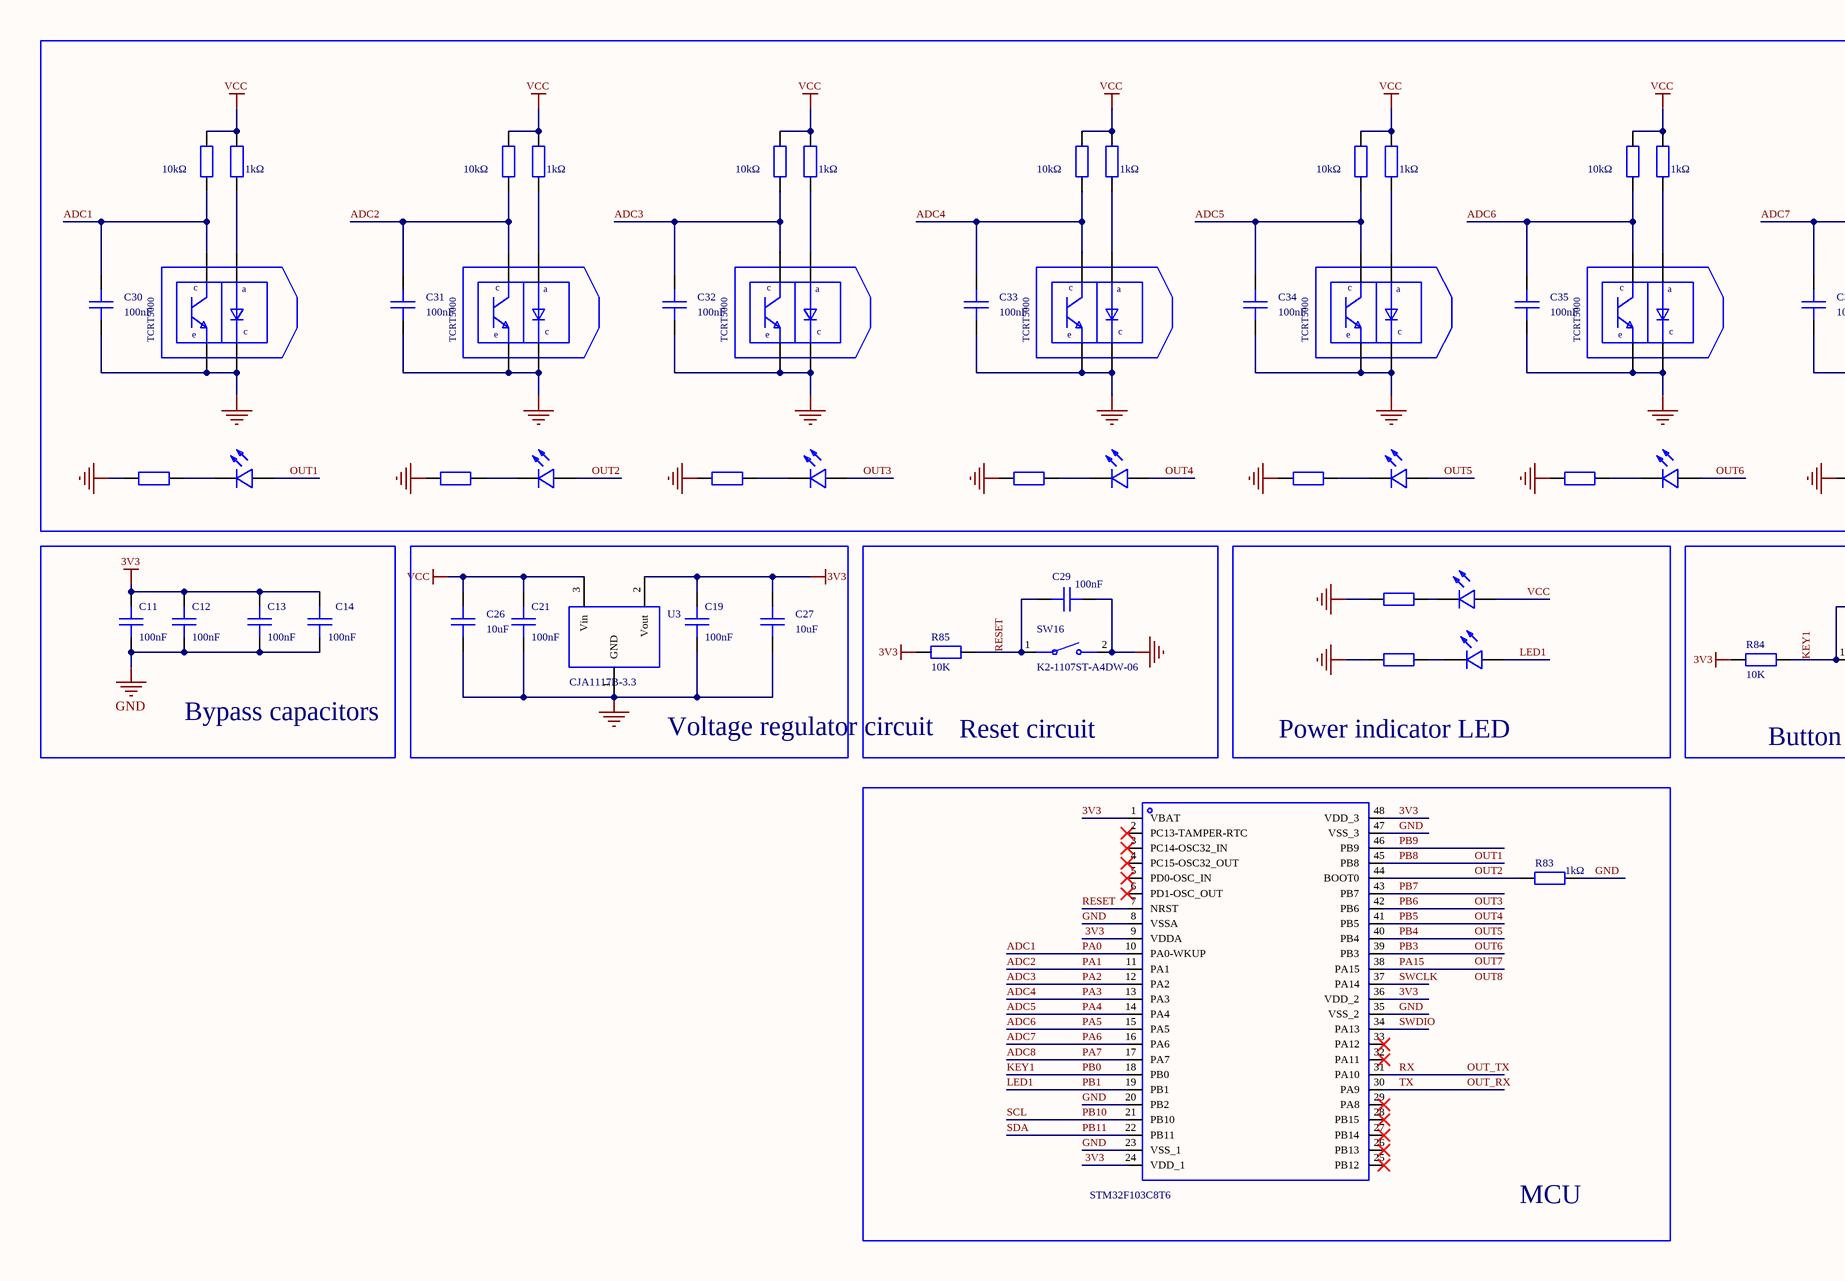
[diagram p0: MISC51279-3.schdoc, left]
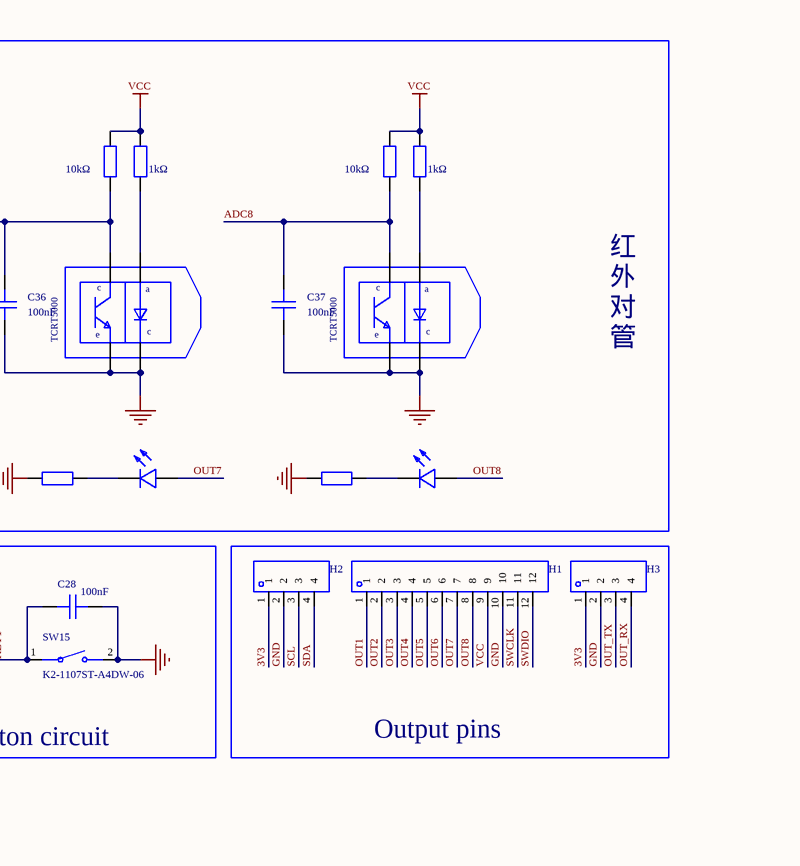
[diagram p1: MISC51279-3.schdoc, right]
# Altium project MISC51279-2.PrjPcb
1 sheet, 72 parts. Net scope: global (net labels, ports and power ports of the same name join across sheets).
Board file: MISC51279.pcbdoc

## Sheet MISC51279-3.schdoc
size 420 x 297 mm; Version: V1.0; @Project Name: MISC51279; @Page Count: 1; @Update Date: 2026-04-29; @Create Date: 2026-04-29; @Schematic Name: MISC51279; @Page No: 1; @Create Time: 12:08:40; @Update Time: 19:15:19; @Board Name: MISC51279

### Parts
C11  100nF  [C0603]
C12  100nF  [C0603]
C13  100nF  [C0603]
C14  100nF  [C0603]
C19  100nF  [C0603]
C21  100nF  [C0603]
C26  10uF  [C0603]
C27  10uF  [C0603]
C28  100nF  [C0603]
C29  100nF  [C0603]
C30  100nF  [C0603]
C31  100nF  [C0603]
C32  100nF  [C0603]
C33  100nF  [C0603]
C34  100nF  [C0603]
C35  100nF  [C0603]
C36  100nF  [C0603]
C37  100nF  [C0603]
CGQ1  TCRT5000L  [OPTO-TH_TCRT5000L]  (value not drawn)
CGQ2  TCRT5000L  [OPTO-TH_TCRT5000L]  (value not drawn)
CGQ3  TCRT5000L  [OPTO-TH_TCRT5000L]  (value not drawn)
CGQ4  TCRT5000L  [OPTO-TH_TCRT5000L]  (value not drawn)
CGQ5  TCRT5000L  [OPTO-TH_TCRT5000L]  (value not drawn)
CGQ6  TCRT5000L  [OPTO-TH_TCRT5000L]  (value not drawn)
CGQ7  TCRT5000L  [OPTO-TH_TCRT5000L]  (value not drawn)
CGQ8  TCRT5000L  [OPTO-TH_TCRT5000L]  (value not drawn)
H1  (no value)  [HDR-TH_12P-P2.54-V-F]
H2  (no value)  [HDR-TH_4P-P2.54-V-F]
H3  (no value)  [HDR-TH_4P-P2.54-V-F]
LED1  NCD0603R1_C84263  [LED0603-RD_RED]  (value not drawn)
LED2  NCD0603R1_C84263  [LED0603-RD_RED]  (value not drawn)
LED3  NCD0603R1_C84263  [LED0603-RD_RED]  (value not drawn)
LED4  NCD0603R1_C84263  [LED0603-RD_RED]  (value not drawn)
LED5  NCD0603R1_C84263  [LED0603-RD_RED]  (value not drawn)
LED6  NCD0603R1_C84263  [LED0603-RD_RED]  (value not drawn)
LED7  NCD0603R1_C84263  [LED0603-RD_RED]  (value not drawn)
LED8  NCD0603R1_C84263  [LED0603-RD_RED]  (value not drawn)
LED9  NCD0603R1_C84263  [LED0603-RD_RED]  (value not drawn)
LED10  NCD0603R1_C84263  [LED0603-RD_RED]  (value not drawn)
R1  value 10kΩ  [R0603]  (hidden comment: 0603WAF1002T5E)
R2  value 1kΩ  [R0603]  (hidden comment: 0603WAF1001T5E)
R3  0603WAF1001T5E  [R0603]  (value not drawn)
R4  value 10kΩ  [R0603]  (hidden comment: 0603WAF1002T5E)
R5  value 1kΩ  [R0603]  (hidden comment: 0603WAF1001T5E)
R6  0603WAF1001T5E  [R0603]  (value not drawn)
R7  value 10kΩ  [R0603]  (hidden comment: 0603WAF1002T5E)
R8  value 1kΩ  [R0603]  (hidden comment: 0603WAF1001T5E)
R9  0603WAF1001T5E  [R0603]  (value not drawn)
R10  value 10kΩ  [R0603]  (hidden comment: 0603WAF1002T5E)
R11  value 1kΩ  [R0603]  (hidden comment: 0603WAF1001T5E)
R12  0603WAF1001T5E  [R0603]  (value not drawn)
R13  value 10kΩ  [R0603]  (hidden comment: 0603WAF1002T5E)
R14  value 1kΩ  [R0603]  (hidden comment: 0603WAF1001T5E)
R15  0603WAF1001T5E  [R0603]  (value not drawn)
R16  value 10kΩ  [R0603]  (hidden comment: 0603WAF1002T5E)
R17  value 1kΩ  [R0603]  (hidden comment: 0603WAF1001T5E)
R18  0603WAF1001T5E  [R0603]  (value not drawn)
R19  value 10kΩ  [R0603]  (hidden comment: 0603WAF1002T5E)
R20  value 1kΩ  [R0603]  (hidden comment: 0603WAF1001T5E)
R21  0603WAF1001T5E  [R0603]  (value not drawn)
R22  value 10kΩ  [R0603]  (hidden comment: 0603WAF1002T5E)
R23  value 1kΩ  [R0603]  (hidden comment: 0603WAF1001T5E)
R24  0603WAF1001T5E  [R0603]  (value not drawn)
R83  1kΩ  [R0603]
R84  10K  [R0603]
R85  10K  [R0603]
R86  0603WAF1001T5E  [R0603]  (value not drawn)
R87  0603WAF1001T5E  [R0603]  (value not drawn)
SW15  K2-1107ST-A4DW-06  [KEY-SMD_L6.2-W3.6-LS8.0]
SW16  K2-1107ST-A4DW-06  [KEY-SMD_L6.2-W3.6-LS8.0]
U1  STM32F103C8T6  [LQFP-48_L7.0-W7.0-P0.50-LS9.0-BL]
U3  CJA1117B-3.3  [SOT-89-3_L4.5-W2.5-P1.50-LS4.2-BR]

### Blocks framed on the sheet
Bypass capacitors: C11-C14
Voltage regulator circuit: C19 C21 C26 C27 U3
Reset circuit: C29 R85 SW16
Power indicator LED: LED9 LED10 R86 R87
Button circuit: C28 R84 SW15
Output pins: H1-H3
MCU: R83 U1

### Nets
3V3: C11.2 C12.2 C13.2 C14.2 C19.2 C27.1 H2.1 H3.1 R84.2 R85.2 U1.1(VBAT) U1.9(VDDA) U1.24(VDD_1) U1.36(VDD_2) U1.48(VDD_3) U3.2(Vout)
GND: C11.1 C12.1 C13.1 C14.1 C19.1 C21.1 C26.2 C27.2 C28.1 C29.1 C30.2 C31.2 C32.2 C33.2 C34.2 C35.2 C36.2 C37.2 CGQ1.2(E) CGQ1.4(C) CGQ2.2(E) CGQ2.4(C) CGQ3.2(E) CGQ3.4(C) CGQ4.2(E) CGQ4.4(C) CGQ5.2(E) CGQ5.4(C) CGQ6.2(E) CGQ6.4(C) CGQ7.2(E) CGQ7.4(C) CGQ8.2(E) CGQ8.4(C) H1.10 H2.2 H3.2 R3.2 R6.2 R9.2 R12.2 R15.2 R18.2 R21.2 R24.2 R83.1 R86.2 R87.2 SW15.2 SW16.2 U1.8(VSSA) U1.20(PB2) U1.23(VSS_1) U1.35(VSS_2) U1.47(VSS_3) U3.1(GND)
VCC: C21.2 C26.1 H1.9 LED9.2(A) R1.2 R2.2 R4.2 R5.2 R7.2 R8.2 R10.2 R11.2 R13.2 R14.2 R16.2 R17.2 R19.2 R20.2 R22.2 R23.2 U3.3(Vin)
ADC1: C30.1 CGQ1.1(C) R1.1 U1.10(PA0-WKUP)  [also labelled PA0]
ADC2: C31.1 CGQ2.1(C) R4.1 U1.11(PA1)  [also labelled PA1]
ADC3: C32.1 CGQ3.1(C) R7.1 U1.12(PA2)  [also labelled PA2]
ADC4: C33.1 CGQ4.1(C) R10.1 U1.13(PA3)  [also labelled PA3]
ADC5: C34.1 CGQ5.1(C) R13.1 U1.14(PA4)  [also labelled PA4]
ADC6: C35.1 CGQ6.1(C) R16.1 U1.15(PA5)  [also labelled PA5]
ADC7: C36.1 CGQ7.1(C) R19.1 U1.16(PA6)  [also labelled PA6]
ADC8: C37.1 CGQ8.1(C) R22.1 U1.17(PA7)  [also labelled PA7]
KEY1: C28.2 R84.1 SW15.1 U1.18(PB0)  [also labelled PB0]
LED1: LED10.2(A) U1.19(PB1)  [also labelled PB1]
OUT1: H1.1 LED1.2(A) U1.46(PB9)  [also labelled PB9]
OUT2: H1.2 LED2.2(A) U1.45(PB8)  [also labelled PB8]
OUT3: H1.3 LED3.2(A) U1.43(PB7)  [also labelled PB7]
OUT4: H1.4 LED4.2(A) U1.42(PB6)  [also labelled PB6]
OUT5: H1.5 LED5.2(A) U1.41(PB5)  [also labelled PB5]
OUT6: H1.6 LED6.2(A) U1.40(PB4)  [also labelled PB4]
OUT7: H1.7 LED7.2(A) U1.39(PB3)  [also labelled PB3]
OUT8: H1.8 LED8.2(A) U1.38(PA15)  [also labelled PA15]
OUT_RX: H3.4 U1.30(PA9)  [also labelled TX]
OUT_TX: H3.3 U1.31(PA10)  [also labelled RX]
PB10: H2.3 U1.21(PB10)  [also labelled SCL]
PB11: H2.4 U1.22(PB11)  [also labelled SDA]
RESET: C29.2 R85.1 SW16.1 U1.7(NRST)
SWCLK: H1.11 U1.37(PA14)
SWDIO: H1.12 U1.34(PA13)
NetCGQ1_3: CGQ1.3(A) R2.1
NetCGQ2_3: CGQ2.3(A) R5.1
NetCGQ3_3: CGQ3.3(A) R8.1
NetCGQ4_3: CGQ4.3(A) R11.1
NetCGQ5_3: CGQ5.3(A) R14.1
NetCGQ6_3: CGQ6.3(A) R17.1
NetCGQ7_3: CGQ7.3(A) R20.1
NetCGQ8_3: CGQ8.3(A) R23.1
NetLED1_1: LED1.1(K) R3.1
NetLED2_1: LED2.1(K) R6.1
NetLED3_1: LED3.1(K) R9.1
NetLED4_1: LED4.1(K) R12.1
NetLED5_1: LED5.1(K) R15.1
NetLED6_1: LED6.1(K) R18.1
NetLED7_1: LED7.1(K) R21.1
NetLED8_1: LED8.1(K) R24.1
NetLED9_1: LED9.1(K) R86.1
NetLED10_1: LED10.1(K) R87.1
NetR83_2: R83.2 U1.44(BOOT0)

Not connected (* = marked no-connect by the designer): U1 2(PC13-TAMPER-RTC)* 3(PC14-OSC32_IN)* 4(PC15-OSC32_OUT)* 5(PD0-OSC_IN)* 6(PD1-OSC_OUT)* 25(PB12)* 26(PB13)* 27(PB14)* 28(PB15)* 29(PA8)* 32(PA11)* 33(PA12)*

### Notes on the sheet
- 红
  外
  对
  管
- 2026-04-29
- Schematic
- Board
- Sheet
- P1
- Drawn
- Reviewed
- Revision
- Size
- A4
- page 1 Total 1

### Library data of the parts
C11-C14 C19 C21 C30-C37 = CAP_0805: ConvertToPcb: yes; SymbolName: CapAcitance; ModelId: 1ba041120af144c991958decab20d241; ModelName: C0805_L2.0-W1.3-H1.3; ModelTransform: 78.74,51.181,0,0,0,0,0,0.0005,0; Device: CAP_0805; AddInBom: yes; Supplier Footprint: 0805; FootprintName: C0603; Value: 100nF
C26 C27 = GRM21BR61H106KE43L: Capacitance: 10uF; tolerance: ±10%; rated voltage: 50V; dielectric (temperature coefficient): X5R;; Manufacturer: muRata(村田); AddInBom: yes; ModelId: 1ba041120af144c991958decab20d241; ModelName: C0805_L2.0-W1.3-H1.3; ModelTransform: 78.74,51.181,0,0,0,0,0,0.0005,0; Symbol: GRM21BR61H106KE43L; Device: GRM21BR61H106KE43L; LCSC Part Name: 10uF ±10% 50V; SupplierPart: C440198; ManufacturerPart: GRM21BR61H106KE43L; Supplier Footprint: 0805; JLCPCB Part Class: Basic library; Datasheet: https://atta.szlcsc.com/upload/public/pdf/source/20230811/95AAE0C9AF55EDC31B7A4D8B733F534E.pdf; Supplier: LCSC; ConvertToPcb: yes; FootprintName: C0603; Value: 10uF; Tolerance: ±10%; Voltage Rated: 50V; Temperature Coefficient: X5R
C28 C29 = CAP_0805: Symbol: CapAcitance; ConvertToPcb: yes; ModelId: 1ba041120af144c991958decab20d241; ModelName: C0805_L2.0-W1.3-H1.3; ModelTransform: 78.74,51.181,0,0,0,0,0,0.0005,0; Device: CAP_0805; AddInBom: yes; Supplier Footprint: 0805; FootprintName: C0603; Value: 100nF
CGQ1-CGQ8 = TCRT5000L: Manufacturer: VISHAY(威世); AddInBom: yes; ModelId: 50930405bf9846238f24432677795c9e; ModelTransform: 401.574,267.716,0,0,0,0,0,0,-133.858; Symbol: TCRT5000L; Device: TCRT5000L; LCSC Part Name: TCRT5000L; SupplierPart: C24085; ManufacturerPart: TCRT5000L; Supplier Footprint: 插件; JLCPCB Part Class: Extended library; Datasheet: https://atta.szlcsc.com/upload/public/pdf/source/20150821/1457707346389.pdf; Supplier: LCSC; ConvertToPcb: yes; FootprintName: OPTO-TH_TCRT5000L; ModelName: OPTO-TH_TCRT5000L
H1 = HDR-F_2.54_1x12P: ConvertToPcb: yes; ModelId: a8b4b2347edc4eeab5667ae97bf18e17; ModelName: HDR-TH_12P-P2.54-F-LI-1X12P; ModelTransform: 1215.74568,98.425,0,0,0,0,0,0,-129.921; Device: HDR-F_2.54_1x12P; Symbol: HDR-F_2.54_1x12P; AddInBom: yes; SupplierPart: C2905419; Supplier Footprint: 插件; FootprintName: HDR-TH_12P-P2.54-V-F
H2 H3 = HDR-F_2.54_1x4P: Symbol: 2.54-1*4P female; ConvertToPcb: yes; ModelId: d187812051054f85879fcaa51a310d8e; ModelTransform: 419.6842,98.464,0,0,0,0,0,0,-118.11; Device: HDR-F_2.54_1x4P; AddInBom: yes; SupplierPart: C2718488; Supplier Footprint: 插件; FootprintName: HDR-TH_4P-P2.54-V-F; ModelName: HDR-TH_4P-P2.54-V-F
LED1-LED10 = NCD0603R1_C84263: 灯头类型:-;发光颜色:红色;正向压降(Vf):1.6V~2.6V;功率:65mW;正向电流:25mA;波长:615nm~630nm;二极管配置:独立二极管;透镜颜色:-;色温:-;发光强度:80mcd~220mcd;发光角度:130°;载带方式:-;工作温度:-30℃~+85℃;; Manufacturer: 国星光电; Symbol: FC-DA1608HRK-620D; AddInBom: yes; ModelId: 74041d3a270d435c8600a9ab9b7641c0; ModelTransform: 63.7794,31.496,0,0,0,0,0,0,0; Illumination Color: Red; Power(Watts): 65mW; Forward Current: 25mA; Diode Configuration: Discrete diode; Viewing Angle: 130°; Device: NCD0603R1_C84263; LCSC Part Name: NCD0603R1; SupplierPart: C84263; ManufacturerPart: NCD0603R1; Supplier Footprint: 0603; JLCPCB Part Class: Extended library; Datasheet: https://atta.szlcsc.com/upload/public/pdf/source/20200820/C84263_DABC6A75E58F576973B407FDBA283D60.pdf; Supplier: LCSC; ConvertToPcb: yes; FootprintName: LED0603-RD_RED; ModelName: LED0603-RD_RED; Lamp Holder Type: -; Voltage - Forward(Vf): 1.6V~2.6V; Wavelength - Dominant: 615nm~630nm; Peak Wavelength: -; Lens Color: -; Color Temperature: -; Luminous Intensity: 80mcd~220mcd; Mounting Sytle: -; Operating Temperature: -30℃~+85℃
R1 R4 R7 R10 R13 R16 R19 R22 = 0603WAF1002T5E: Type: thick-film resistor; resistance: 10kΩ; tolerance: ±1%; power: 100mW; max working voltage: 75V; temperature coefficient: ±100ppm/°C;; Manufacturer: UNI-ROYAL(厚声); AddInBom: yes; ModelId: fc143cca1e79419f9cd78b61e9279f08; ModelTransform: 31.8897,63.7794,0,90,0,0,0,0,0; Temperature Coefficient: ±100ppm/℃; Symbol: 0603WAF1002T5E; Device: 0603WAF1002T5E; LCSC Part Name: 厚膜电阻 10kΩ ±1% 100mW; SupplierPart: C25804; ManufacturerPart: 0603WAF1002T5E; Supplier Footprint: 0603; JLCPCB Part Class: Basic library; Datasheet: https://atta.szlcsc.com/upload/public/pdf/source/20200306/C422600_1E6D84923E4A46A82E41ADD87F860B5C.pdf; Supplier: LCSC; ConvertToPcb: yes; FootprintName: R0603; ModelName: R0603; Type: Thick-film resistor; Tolerance: ±1%; Power(Watts): 100mW; Overload Voltage (Max): 75V; Operating Temperature Range: -55℃~+155℃
R2 R3 R5 R6 R8 R9 R11 R12 R14 R15 R17 R18 R20 R21 R23 R24 R86 R87 = 0603WAF1001T5E: Type: thick-film resistor; resistance: 1kΩ; tolerance: ±1%; power: 100mW; max working voltage: 75V; temperature coefficient: ±100ppm/°C;; Manufacturer: UNI-ROYAL(厚声); AddInBom: yes; ModelId: fc143cca1e79419f9cd78b61e9279f08; ModelTransform: 31.8897,63.7794,0,90,0,0,0,0,0; Temperature Coefficient: ±100ppm/℃; Symbol: 0603WAF1001T5E; Device: 0603WAF1001T5E; LCSC Part Name: 1kΩ ±1% 100mW 厚膜电阻; SupplierPart: C21190; ManufacturerPart: 0603WAF1001T5E; Supplier Footprint: 0603; JLCPCB Part Class: Basic library; Datasheet: https://atta.szlcsc.com/upload/public/pdf/source/20200306/C422600_1E6D84923E4A46A82E41ADD87F860B5C.pdf; Supplier: LCSC; ConvertToPcb: yes; FootprintName: R0603; ModelName: R0603; Type: Thick-film resistor; Tolerance: ±1%; Power(Watts): 100mW; Overload Voltage (Max): 75V; Operating Temperature Range: -55℃~+155℃
  R3 R6 R9 R12 R15 R18 R21 R24 R86 R87: Value: 1kΩ
R83 = 0805W8F1001T5E: Type: thick-film resistor; resistance: 1kΩ; tolerance: ±1%; power: 125mW; max working voltage: 150V; temperature coefficient: ±100ppm/°C;; Manufacturer: UNI-ROYAL(厚声); AddInBom: yes; ModelId: 37a81e68749a4138bd2dfa6897b24b85; ModelName: R0805_L2.0-W1.3-H0.6; ModelTransform: 78.74,51.181,0,0,0,0,0,-0.0005,0; Temperature Coefficient: ±100ppm/℃; Symbol: 0805W8F1001T5E; Device: 0805W8F1001T5E; LCSC Part Name: 1kΩ ±1% 125mW 厚膜电阻; SupplierPart: C17513; ManufacturerPart: 0805W8F1001T5E; Supplier Footprint: 0805; JLCPCB Part Class: Basic library; Datasheet: https://atta.szlcsc.com/upload/public/pdf/source/20200306/C422600_1E6D84923E4A46A82E41ADD87F860B5C.pdf; Supplier: LCSC; ConvertToPcb: yes; FootprintName: R0603; Type: Thick-film resistor; Value: 1kΩ; Tolerance: ±1%; Power(Watts): 125mW; Overload Voltage (Max): 150V; Operating Temperature Range: -55℃~+155℃
R84 R85 = Res_0805: Symbol: Resistor; ConvertToPcb: yes; ModelId: 37a81e68749a4138bd2dfa6897b24b85; ModelName: R0805_L2.0-W1.3-H0.6; ModelTransform: 78.74,51.181,0,0,0,0,0,-0.0005,0; Device: Res_0805; AddInBom: yes; Supplier Footprint: 0805; Value: 10K; FootprintName: R0603
SW15 SW16 = K2-1107ST-A4DW-06: 电路结构:单刀单掷;按钮形状:矩形按钮;作用力:250gf;安装方式:立贴;开关长度:6.1mm;开关宽度:3.6mm;开关高度:2.5mm;触点电流:50mA;额定电压(DC):12V;绝缘电阻:100MΩ;带灯:-;机械寿命:10万次;; Manufacturer: 韩国韩荣; Symbol: K2-1107ST-A4SW-06; AddInBom: yes; ModelId: 4e4c8eb7a320436abebac0b9b4254e2e; ModelName: KEY-SMD_2P-L6.2-W3.6-LS8.0; ModelTransform: 311.023,141.732,0,0,0,0,0,-0.001,0; Circuit: SPST; Actuator Style: Rectangular button; Operating Force: 250gf; Switch Length: 6.1mm; Switch Width: 3.6mm; Switch Height: 2.5mm; Contact Current: 50mA; Voltage Rating (DC): 12V; Insulation Resistance: 100MΩ; Mechanical Life: 10万 cycles; Device: K2-1107ST-A4DW-06; LCSC Part Name: 轻触开关 3.6*6.1*2.5; SupplierPart: C118141; ManufacturerPart: K2-1107ST-A4DW-06; Supplier Footprint: SMD; JLCPCB Part Class: Extended library; Datasheet: https://atta.szlcsc.com/upload/public/pdf/source/20210810/381712CEF248770C072B585C3485C888.pdf; Supplier: LCSC; ConvertToPcb: yes; FootprintName: KEY-SMD_L6.2-W3.6-LS8.0; Mounting Style: Vertical SMD; With Lamp: -; Operating Temperature: -25℃~+85℃
U1 = STM32F103C8T6: CPU core: ARM Cortex-M3; CPU max clock: 72MHz; program memory capacity: 64KB; program memory type: FLASH; total RAM: 20KB; GPIO port count: 37;; Manufacturer: ST(意法半导体); AddInBom: yes; ModelId: 093be70396ff421eb2cdb946d5311efc; ModelName: LQFP-48_L7.0-W7.0-H1.4-LS9.0-P0.50; ModelTransform: 354.331,354.331,0,0,0,0,0,0,0; Operating Voltage Range: 2V~3.6V; GPIO Ports Number: 37; ADC (Bit): 12bit; Peripheral/Function: Watchdog; DMA; Watchdog; On-chip temperature sensor; Device: STM32F103C8T6; Symbol: STM32F103C8T6; LCSC Part Name: ARM Cortex-M3 72MHz MSL=3; SupplierPart: C8734; ManufacturerPart: STM32F103C8T6; Supplier Footprint: LQFP-48(7x7); JLCPCB Part Class: Basic library; Datasheet: https://atta.szlcsc.com/upload/public/pdf/source/20220812/8363ACEC51AD55ECEB84799464F7CB85.pdf; Supplier: LCSC; ConvertToPcb: yes; FootprintName: LQFP-48_L7.0-W7.0-P0.50-LS9.0-BL; CPU Core: ARM Cortex-M3; CPU Maximum Speed: 72MHz; Program Storage Size: 64KB; Program Memory Type: FLASH; RAM Size: 20KB; EEPROM: -; DAC (Bit): -; PWM (Bit): -; Universal Serial Bus: Yes; Internal Comparator: -; communication protocol: -; Watchdog: Yes; Real-Time Clock: -; Infrared Data Association: Yes; Low-Voltage Detect: Yes; CCP Capture/Compare: -; Secure Digital Input and Output: -; Direct Memory Access: Yes; Internal Oscillator: Yes; Operating Temperature Range: -40℃~+85℃
U3 = CJA1117B-3.3: Output type: fixed; max input voltage: 15V; output voltage: 3.3V; max output current: 1A; ripple rejection (PSRR): 75dB@(120Hz); output polarity: positive;; Manufacturer: CJ(江苏长电/长晶); AddInBom: yes; ModelId: 6db690b7897d4d18a30d90c1b89525ee; ModelName: SOT-89-3_L4.3-W2.5-H1.6-LS4.1-P1.50; ModelTransform: 161.417,169.291,0,180,0,0,-11.808,0,0; Dropout Voltage: 1.3V@(1A); Number of Outputs: 1; Symbol: CJA1117B-3.3; Device: CJA1117B-3.3; Supplier: LCSC; Manufacturer Part: CJA1117B-3.3; Supplier Part: C24253; JLCPCB Part Class: Extended library; LCSC Part Name: 输入15V 输出3.3V 1A; Supplier Footprint: SOT-89-3; Datasheet: https://atta.szlcsc.com/upload/public/pdf/source/20170719/C107222_1500457721357828222.pdf; ConvertToPcb: yes; FootprintName: SOT-89-3_L4.5-W2.5-P1.50-LS4.2-BR; Output Type: Fixed; Maximum Input Voltage: 15V; Output Voltage: 3.3V; MAX Output Current: 1A; Power Supply Rejection Ratio (PSRR): 75dB@(120Hz); Output Polarity: Positive